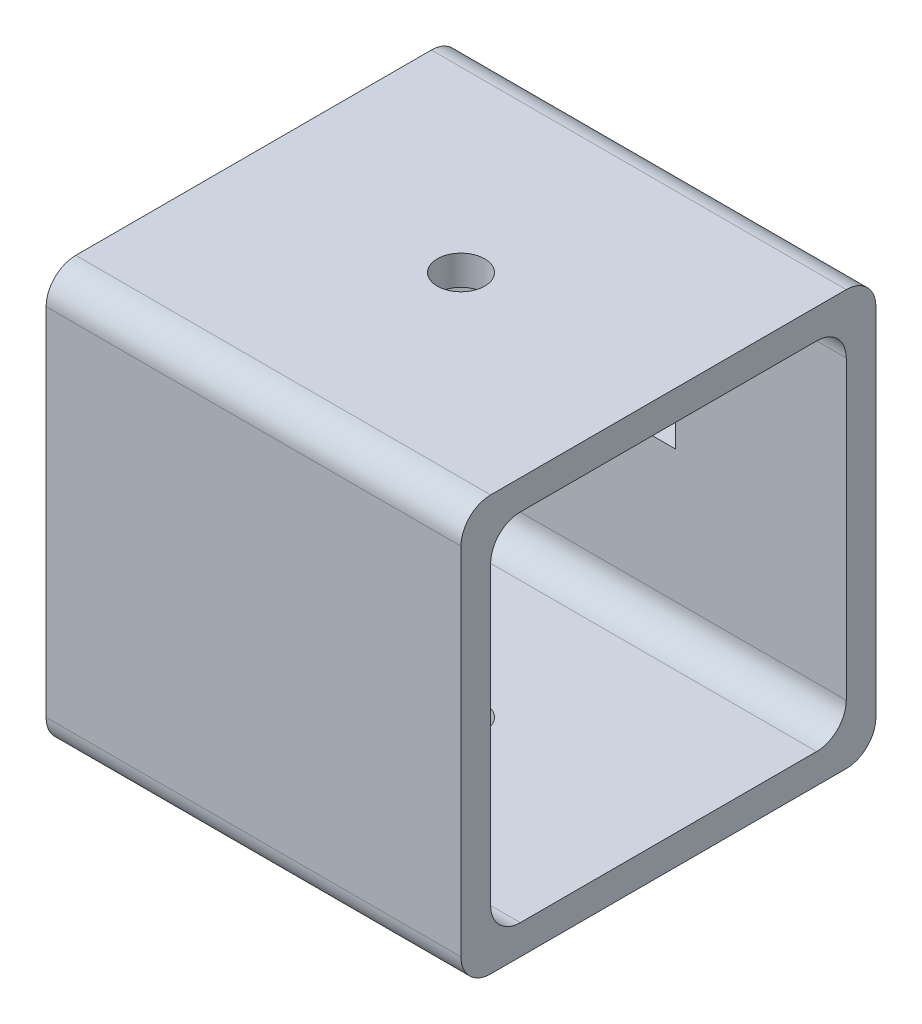
SolidWorks part; units mm, degrees
ref_plane "Front Plane" through (0, 0, 0) normal (0, 0, 1) x (1, 0, 0)
ref_plane "Top Plane" through (0, 0, 0) normal (0, 1, 0) x (1, 0, 0)
ref_plane "Right Plane" through (0, 0, 0) normal (1, 0, 0) x (0, 0, -1)
sketch "Sketch1" plane through (0, 0, 0) normal (0, 0, 1) x (1, 0, 0)
  line L1 (35, 35) -> (-35, 35)
  line L2 (35, 35) -> (35, -35)
  line L3 (35, -35) -> (-35, -35)
  line L4 (-35, 35) -> (-35, -35)
  line L5 (35, 35) -> (-35, -35) construction
  line L6 (35, -35) -> (-35, 35) construction
  point P0 (0, 0)
  dimension "D1" = 70
  dimension "D2" = 70
extrude "Boss-Extrude1" add sketch "Sketch1" along normal blind 70
sketch "Sketch2" plane through (35, 0, 0) normal (1, 0, 0) x (0, 0, -1)
  line L8 (-5, -30) -> (-5, 30)
  line L9 (-5, 30) -> (-65, 30)
  line L10 (-65, 30) -> (-65, -30)
  line L11 (-65, -30) -> (-5, -30)
  line L12 (-5, -30) -> (-5, 30)
  line L13 (-5, 30) -> (-65, 30)
  line L14 (-65, 30) -> (-65, -30)
  line L15 (-65, -30) -> (-5, -30)
  dimension "D1" = 5
extrude "Cut-Extrude1" cut sketch "Sketch2" against normal blind 104
sketch "Sketch3" plane through (0, 0, 0) normal (0, 0, -1) x (-1, 0, 0)
  line L1 (6.2, 2.7) -> (-6.2, 2.7)
  line L2 (6.2, 2.7) -> (6.2, -2.7)
  line L3 (6.2, -2.7) -> (-6.2, -2.7)
  line L4 (-6.2, 2.7) -> (-6.2, -2.7)
  line L5 (6.2, 2.7) -> (-6.2, -2.7) construction
  line L6 (6.2, -2.7) -> (-6.2, 2.7) construction
  point P0 (0, 0)
  dimension "D1" = 5.4
  dimension "D2" = 12.4
extrude "Cut-Extrude2" cut sketch "Sketch3" against normal blind 10
sketch "Sketch4" plane through (0, -35, 0) normal (0, -1, 0) x (1, 0, 0)
  line L0 (0, 70) -> (0, 0) construction
  line L1 (-35, 70) -> (35, 70) construction
  circle A0 centre (0, 35) radius 4
  dimension "D1" = 8
extrude "Cut-Extrude3" cut sketch "Sketch4" against normal blind 122
fillet "Fillet1" radius 5 8 edges at (0, 35, 70) (0, -35, 70) (0, 30, 65) (0, -30, 65) (0, -30, 5) (0, 30, 5) (0, 35, 0) (0, -35, 0)
